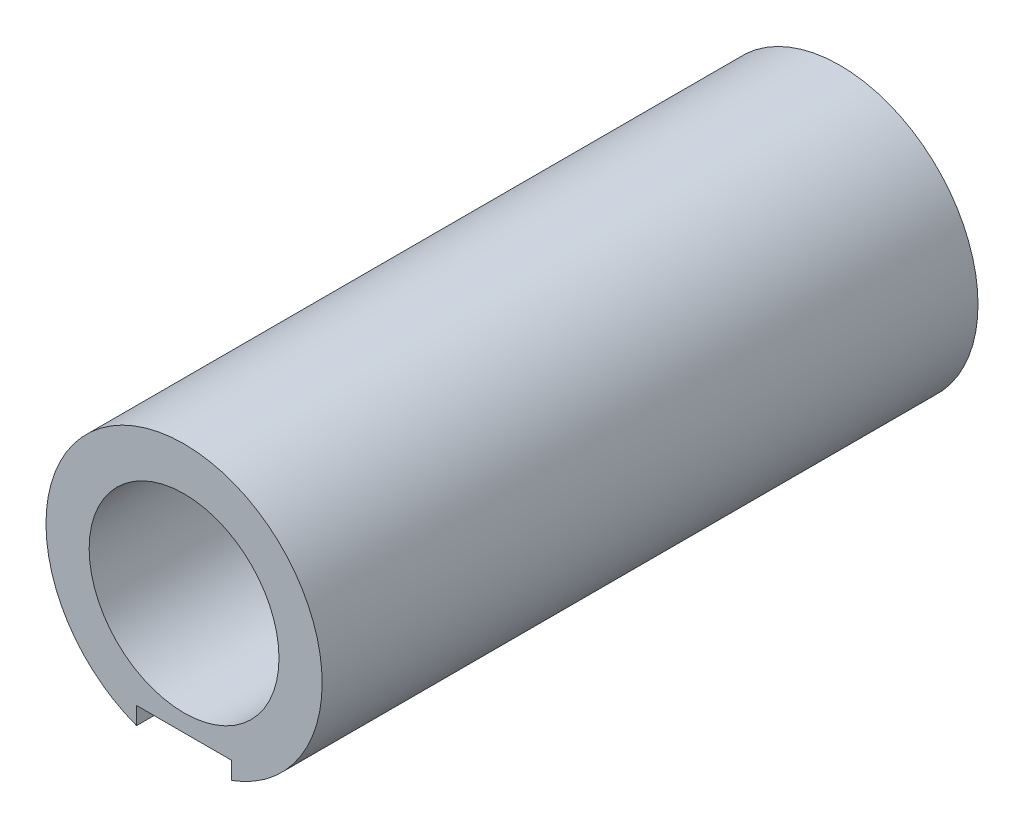
from build123d import *

# Parameters (mm, degrees)
SKETCH1_R               = 80
BOSS_EXTRUDE1_DEPTH     = 380
CUT_EXTRUDE1_START      = -97
CUT_EXTRUDE1_DEPTH      = 97
CUT_EXTRUDE2_DEPTH      = 798.2092078
CUT_EXTRUDE2_DEPTH_BACK = 798.2092078
SKETCH3_R               = 55


with BuildPart() as part:
    # Sketch1 → Boss-Extrude1 (new body)
    with BuildSketch(Plane.XY):
        with Locations((-599.884196758, -90)):
            Circle(SKETCH1_R)
    extrude(amount=BOSS_EXTRUDE1_DEPTH)

    # Sketch2 → Cut-Extrude1 (cut)
    with BuildSketch(Plane.XY.offset(380).offset(CUT_EXTRUDE1_START)):
        with BuildLine():
            ThreePointArc((-627.384196758, -165.124896007), (-599.884196758, -170), (-572.384196758, -165.124896007))
            Line((-572.384196758, -165.124896007), (-572.384196758, -155))
            Line((-572.384196758, -155), (-627.384196758, -155))
            Line((-627.384196758, -155), (-627.384196758, -165.124896007))
        make_face()
    extrude(amount=CUT_EXTRUDE1_DEPTH, mode=Mode.SUBTRACT)

    # Sketch3 → Cut-Extrude2 (cut, two sides: drawn at the far end of the back side and taken through both)
    with BuildSketch(Plane.XY.offset(380).offset(-CUT_EXTRUDE2_DEPTH_BACK)):
        with Locations((-599.884196758, -90)):
            Circle(SKETCH3_R)
    extrude(amount=CUT_EXTRUDE2_DEPTH + CUT_EXTRUDE2_DEPTH_BACK, mode=Mode.SUBTRACT)


solid = part.part
